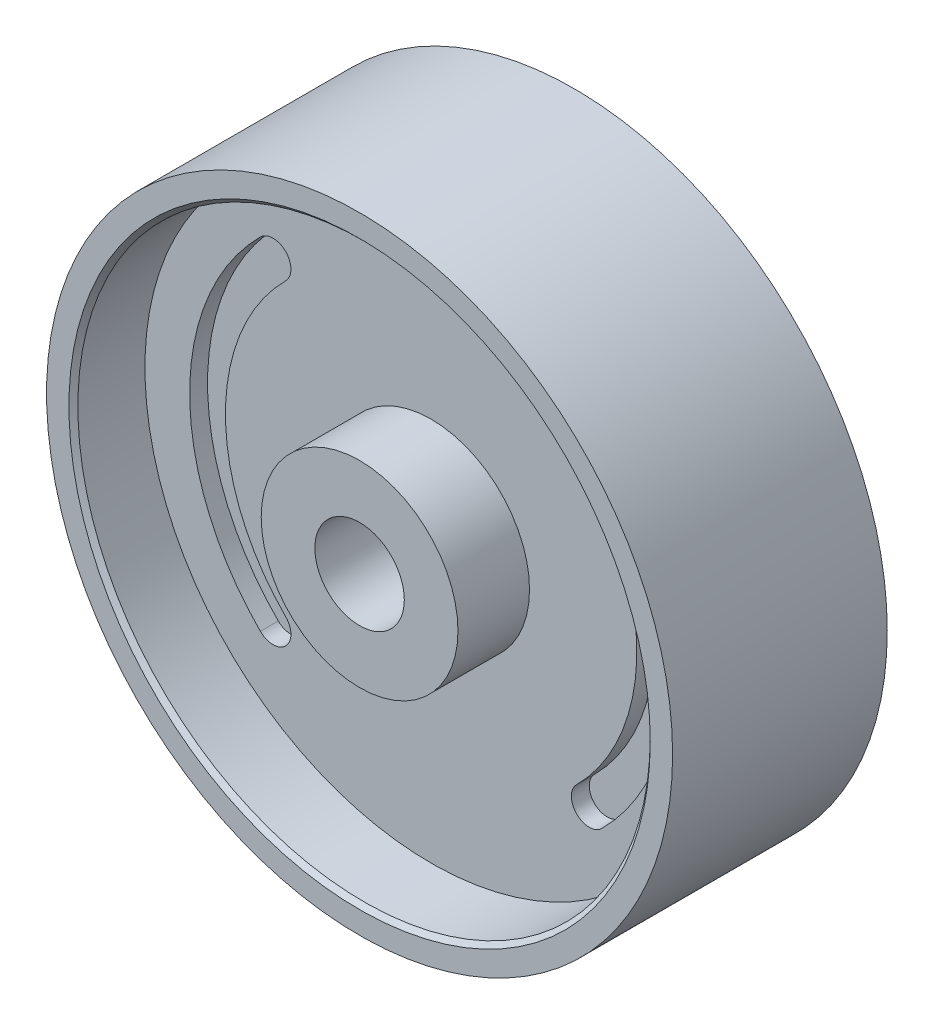
from build123d import *

# Parameters (mm, degrees)
SKETCH1_R           = 35
BOSS_EXTRUDE1_DEPTH = 12
SKETCH2_R           = 5
CUT_EXTRUDE1_DEPTH  = 70.5
SKETCH3_R           = 32
SKETCH3_R_2         = 11
CUT_EXTRUDE2_DEPTH  = 8
CUT_EXTRUDE3_DEPTH  = 2
CHAMFER1_SIZE       = 0.5


with BuildPart() as part:
    # Sketch1 → Boss-Extrude1 (new, symmetric)
    with BuildSketch(Plane.XY):
        Circle(SKETCH1_R)
    extrude(amount=BOSS_EXTRUDE1_DEPTH, both=True)

    # Sketch2 → Cut-Extrude1 (cut, symmetric)
    with BuildSketch(Plane.XY.offset(12)):
        Circle(SKETCH2_R)
    extrude(amount=CUT_EXTRUDE1_DEPTH, both=True, mode=Mode.SUBTRACT)

    # Sketch3 → Cut-Extrude2 (cut)
    with BuildSketch(Plane.XY.offset(12)):
        Circle(SKETCH3_R)
        Circle(SKETCH3_R_2, mode=Mode.SUBTRACT)
    cut_extrude2 = extrude(amount=-CUT_EXTRUDE2_DEPTH, mode=Mode.SUBTRACT)

    # Mirror1: Cut-Extrude2 across plane
    add(cut_extrude2.mirror(Plane.XY), mode=Mode.SUBTRACT)

    # Sketch4 → Cut-Extrude3 (cut)
    with BuildSketch(Plane(origin=(0, 0, -4), x_dir=(-1, 0, 0), z_dir=(0, 0, -1))):
        with BuildLine():
            ThreePointArc((19.091883092, -19.091883092), (27, 0), (19.091883092, 19.091883092))
            ThreePointArc((19.091883092, 19.091883092), (16.263455967, 19.091883092), (16.263455967, 16.263455967))
            ThreePointArc((16.263455967, 16.263455967), (23, 0), (16.263455967, -16.263455967))
            ThreePointArc((16.263455967, -16.263455967), (16.263455967, -19.091883092), (19.091883092, -19.091883092))
        make_face()
        with BuildLine():
            ThreePointArc((-19.091883092, -19.091883092), (-27, 0), (-19.091883092, 19.091883092))
            ThreePointArc((-19.091883092, 19.091883092), (-16.263455967, 19.091883092), (-16.263455967, 16.263455967))
            ThreePointArc((-16.263455967, 16.263455967), (-23, 0), (-16.263455967, -16.263455967))
            ThreePointArc((-16.263455967, -16.263455967), (-16.263455967, -19.091883092), (-19.091883092, -19.091883092))
        make_face()
    cut_extrude3 = extrude(amount=-CUT_EXTRUDE3_DEPTH, mode=Mode.SUBTRACT)

    # Mirror2: Cut-Extrude3 across plane
    add(cut_extrude3.mirror(Plane.XY), mode=Mode.SUBTRACT)

    # Chamfer1
    chamfer1_edges = [part.edges().sort_by_distance(p)[0] for p in [
        (-32, 0, 12),
        (-32, 0, -12),
    ]]
    chamfer(chamfer1_edges, length=CHAMFER1_SIZE)


solid = part.part
